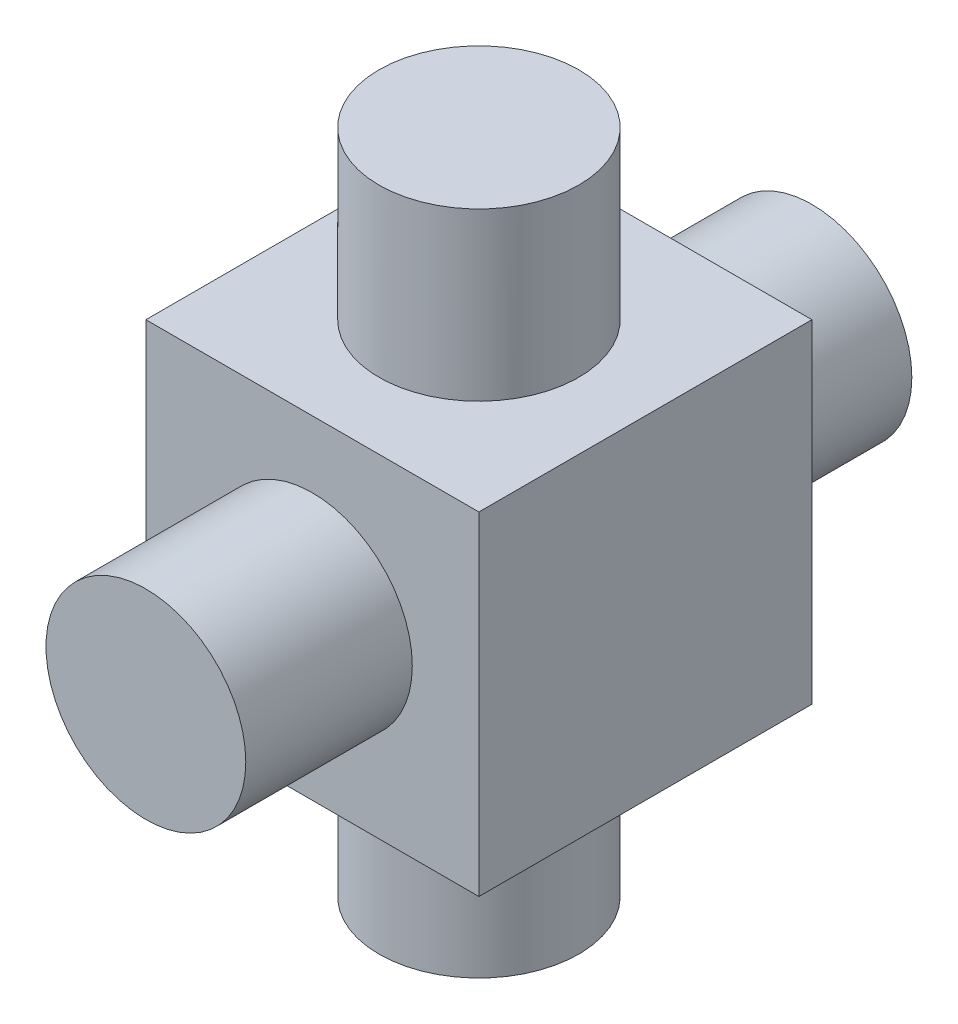
SolidWorks part; units mm, degrees
ref_plane "前视基准面" through (0, 0, 0) normal (0, 0, 1) x (1, 0, 0)
ref_plane "上视基准面" through (0, 0, 0) normal (0, 1, 0) x (1, 0, 0)
ref_plane "右视基准面" through (0, 0, 0) normal (1, 0, 0) x (0, 0, -1)
sketch "草图1" plane through (0, 0, 0) normal (0, 0, 1) x (1, 0, 0)
  line L1 (-2.5, 2.5) -> (2.5, 2.5)
  line L2 (-2.5, 2.5) -> (-2.5, -2.5)
  line L3 (-2.5, -2.5) -> (2.5, -2.5)
  line L4 (2.5, 2.5) -> (2.5, -2.5)
  point P4 (0, 2.5)
  point P6 (-2.5, 0)
  dimension "D1" = 5
  dimension "5" = 5
extrude "凸台-拉伸1" add sketch "草图1" along normal mid plane 5
sketch "草图2" plane through (0, 0, 0) normal (0, 1, 0) x (1, 0, 0)
  circle A0 centre (0, 0) radius 1.5
extrude "凸台-拉伸2" add sketch "草图2" along normal mid plane 10
sketch "草图3" plane through (0, 0, 0) normal (0, 0, 1) x (1, 0, 0)
  circle A0 centre (0, 0) radius 1.5
extrude "凸台-拉伸3" add sketch "草图3" along normal mid plane 10
